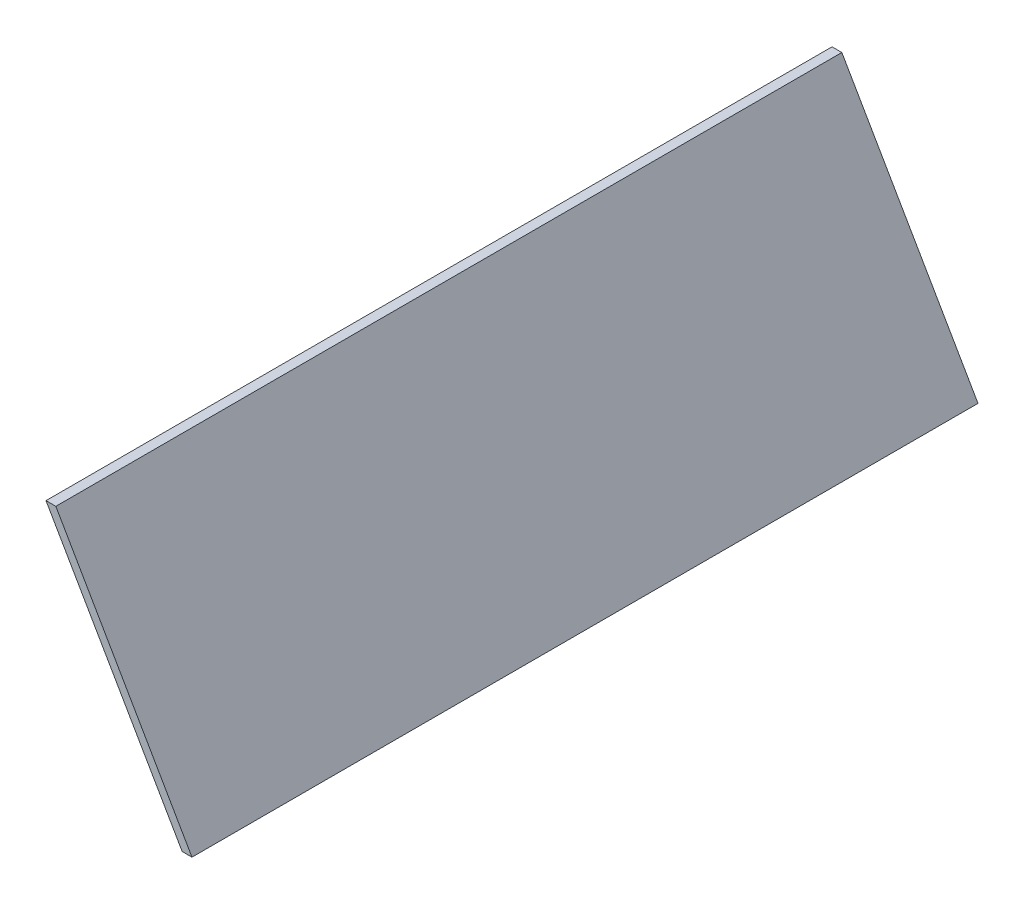
SolidWorks part; units mm, degrees
ref_plane "前视基准面" through (0, 0, 0) normal (0, 0, 1) x (1, 0, 0)
ref_plane "上视基准面" through (0, 0, 0) normal (0, 1, 0) x (1, 0, 0)
ref_plane "右视基准面" through (0, 0, 0) normal (1, 0, 0) x (0, 0, -1)
sketch "草图1" plane through (0, 0, 0) normal (0, 0, 1) x (1, 0, 0)
  line L0 (0, 0) -> (5, 0)
  line L1 (5, 0) -> (74.282, -120)
  line L2 (74.282, -120) -> (69.282, -120)
  line L3 (69.282, -120) -> (0, 0)
  dimension "D1" = 120
  dimension "D2" = 5
  dimension "D3" = 60
extrude "凸台-拉伸1" add sketch "草图1" along normal blind 400
